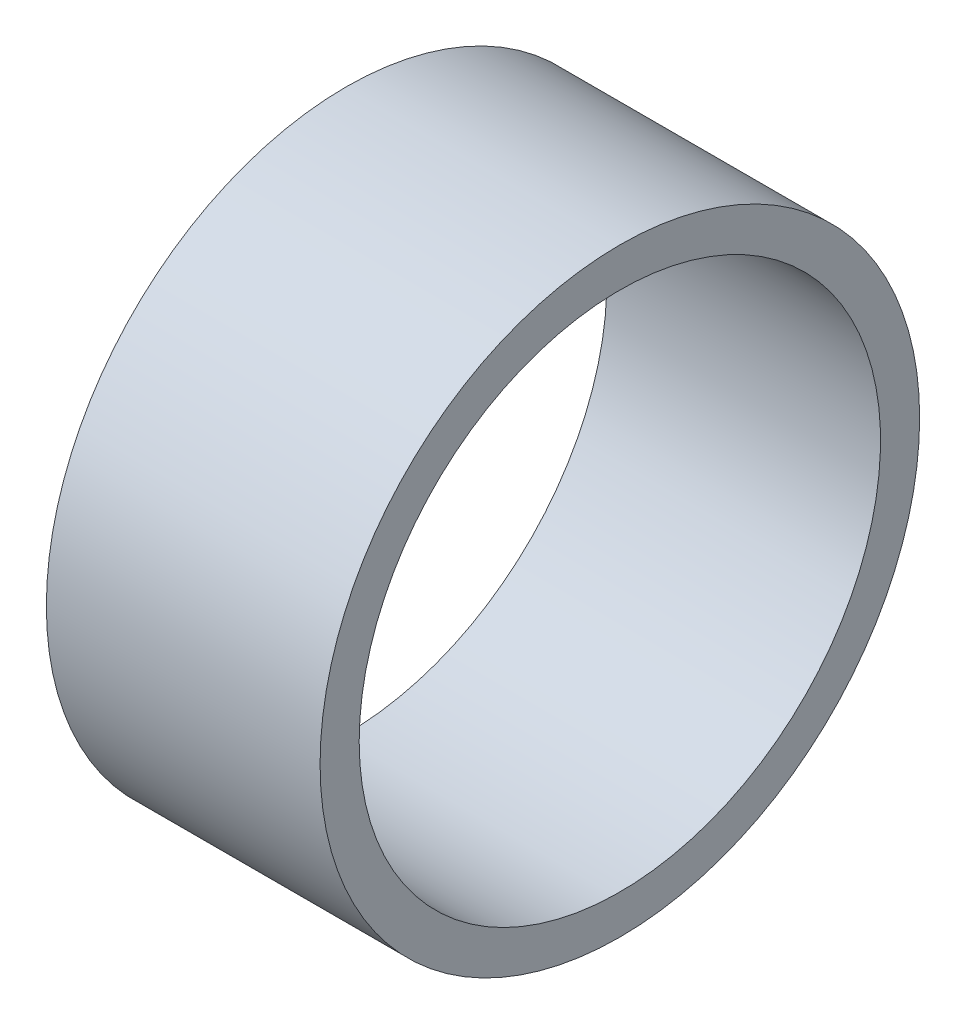
from build123d import *

# Parameters (mm, degrees)
SKETCH_1_R      = 23
SKETCH_1_R_2    = 20
EXTRUDE_1_DEPTH = 21


with BuildPart() as part:
    # 草图1 → 凸台-拉伸1 (new body)
    with BuildSketch(Plane(origin=(0, 0, 0), x_dir=(0, 0, -1), z_dir=(1, 0, 0))):
        with Locations(Location((0, 0, 0), (0, 0, 180))):
            Circle(SKETCH_1_R)
        with Locations(Location((0, 0, 0), (0, 0, 180))):
            Circle(SKETCH_1_R_2, mode=Mode.SUBTRACT)
    extrude(amount=EXTRUDE_1_DEPTH)


solid = part.part
